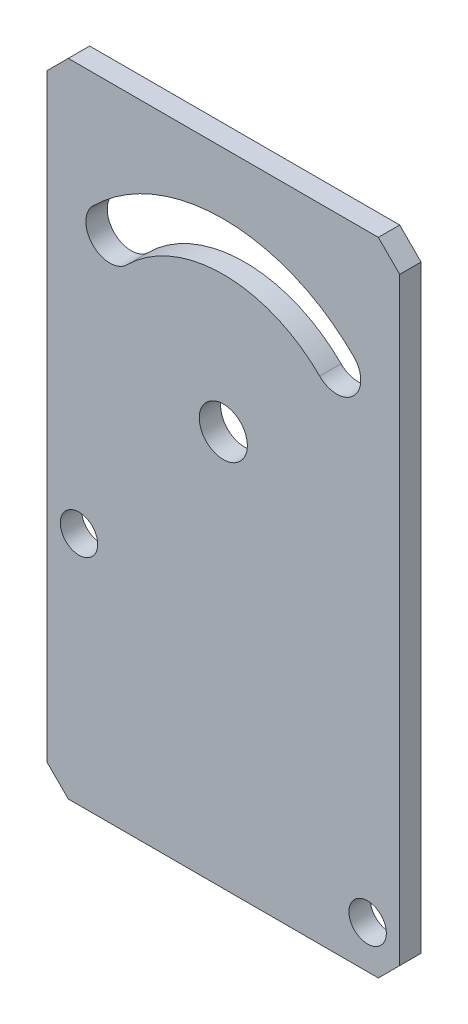
SolidWorks part; units mm, degrees
material "Q235-A"
ref_plane "Front Plane" through (0, 0, 0) normal (0, 0, 1) x (1, 0, 0)
ref_plane "Top Plane" through (0, 0, 0) normal (0, 1, 0) x (1, 0, 0)
ref_plane "Right Plane" through (0, 0, 0) normal (1, 0, 0) x (0, 0, -1)
sketch "Sketch1" plane through (0, 0, 0) normal (0, 0, 1) x (1, 0, 0)
  line L0 (0, 30) -> (0, -30) construction
  line L1 (-16.5, -30) -> (16.5, -30)
  line L2 (-16.5, -30) -> (-16.5, 30)
  line L3 (-16.5, 30) -> (16.5, 30)
  line L4 (16.5, -30) -> (16.5, 30)
  line L5 (-16.5, -30) -> (16.5, 30) construction
  line L6 (-16.5, 30) -> (16.5, -30) construction
  line L7 (0, 7) -> (14.1226, 21.1226) construction
  line L8 (0, 7) -> (-15.4948, 22.4948) construction
  circle A0 centre (0, 7) radius 2.25
  circle A1 centre (13.5, -26) radius 1.75
  circle A2 centre (-13.5, -8) radius 1.75
  circle A3 centre (0, 7) radius 15 construction
  arc A5 (9.0156, 16.0156) -> (-9.0156, 16.0156) centre (0, 7) ccw
  arc A6 (-12.1976, 19.1976) -> (-9.0156, 16.0156) centre (-10.6066, 17.6066) ccw
  arc A7 (9.0156, 16.0156) -> (12.1976, 19.1976) centre (10.6066, 17.6066) ccw
  arc A8 (12.1976, 19.1976) -> (-12.1976, 19.1976) centre (0, 7) ccw
  point P0 (0, 0)
  dimension "D3" = 37
  dimension "D4" = 4
  dimension "D5" = 3
  dimension "D6" = 3.5
  dimension "D7" = 3.5
  dimension "D8" = 27
  dimension "D9" = 18
  dimension "D1" = 33
  dimension "D2" = 60
extrude "Boss-Extrude1" add sketch "Sketch1" along normal blind 2
chamfer "Chamfer1" distance 2 angle 45 4 edges at (16.5, -30, 1) (-16.5, -30, 1) (16.5, 30, 1) (-16.5, 30, 1)
